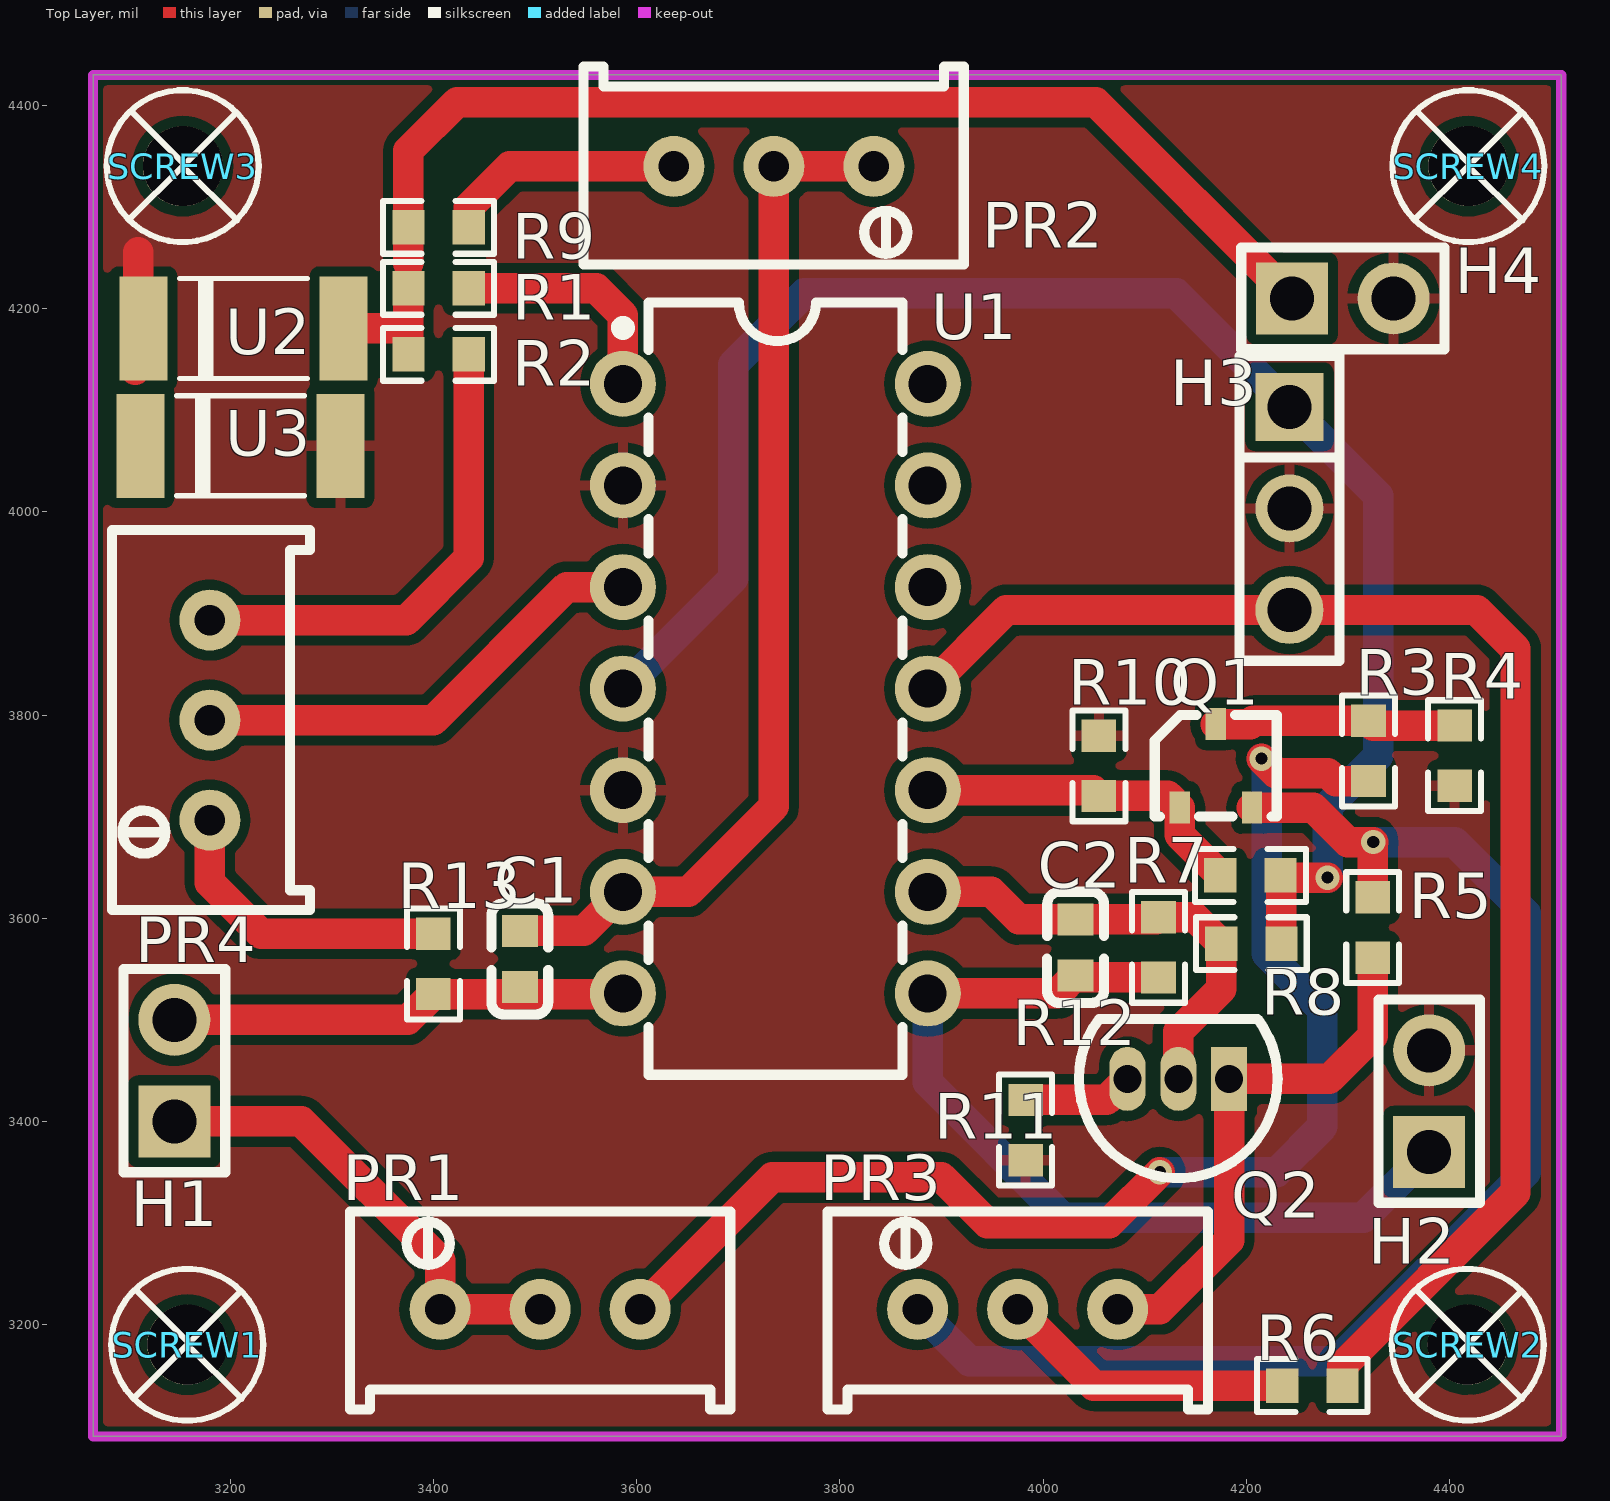
[diagram p0: Top Layer view]
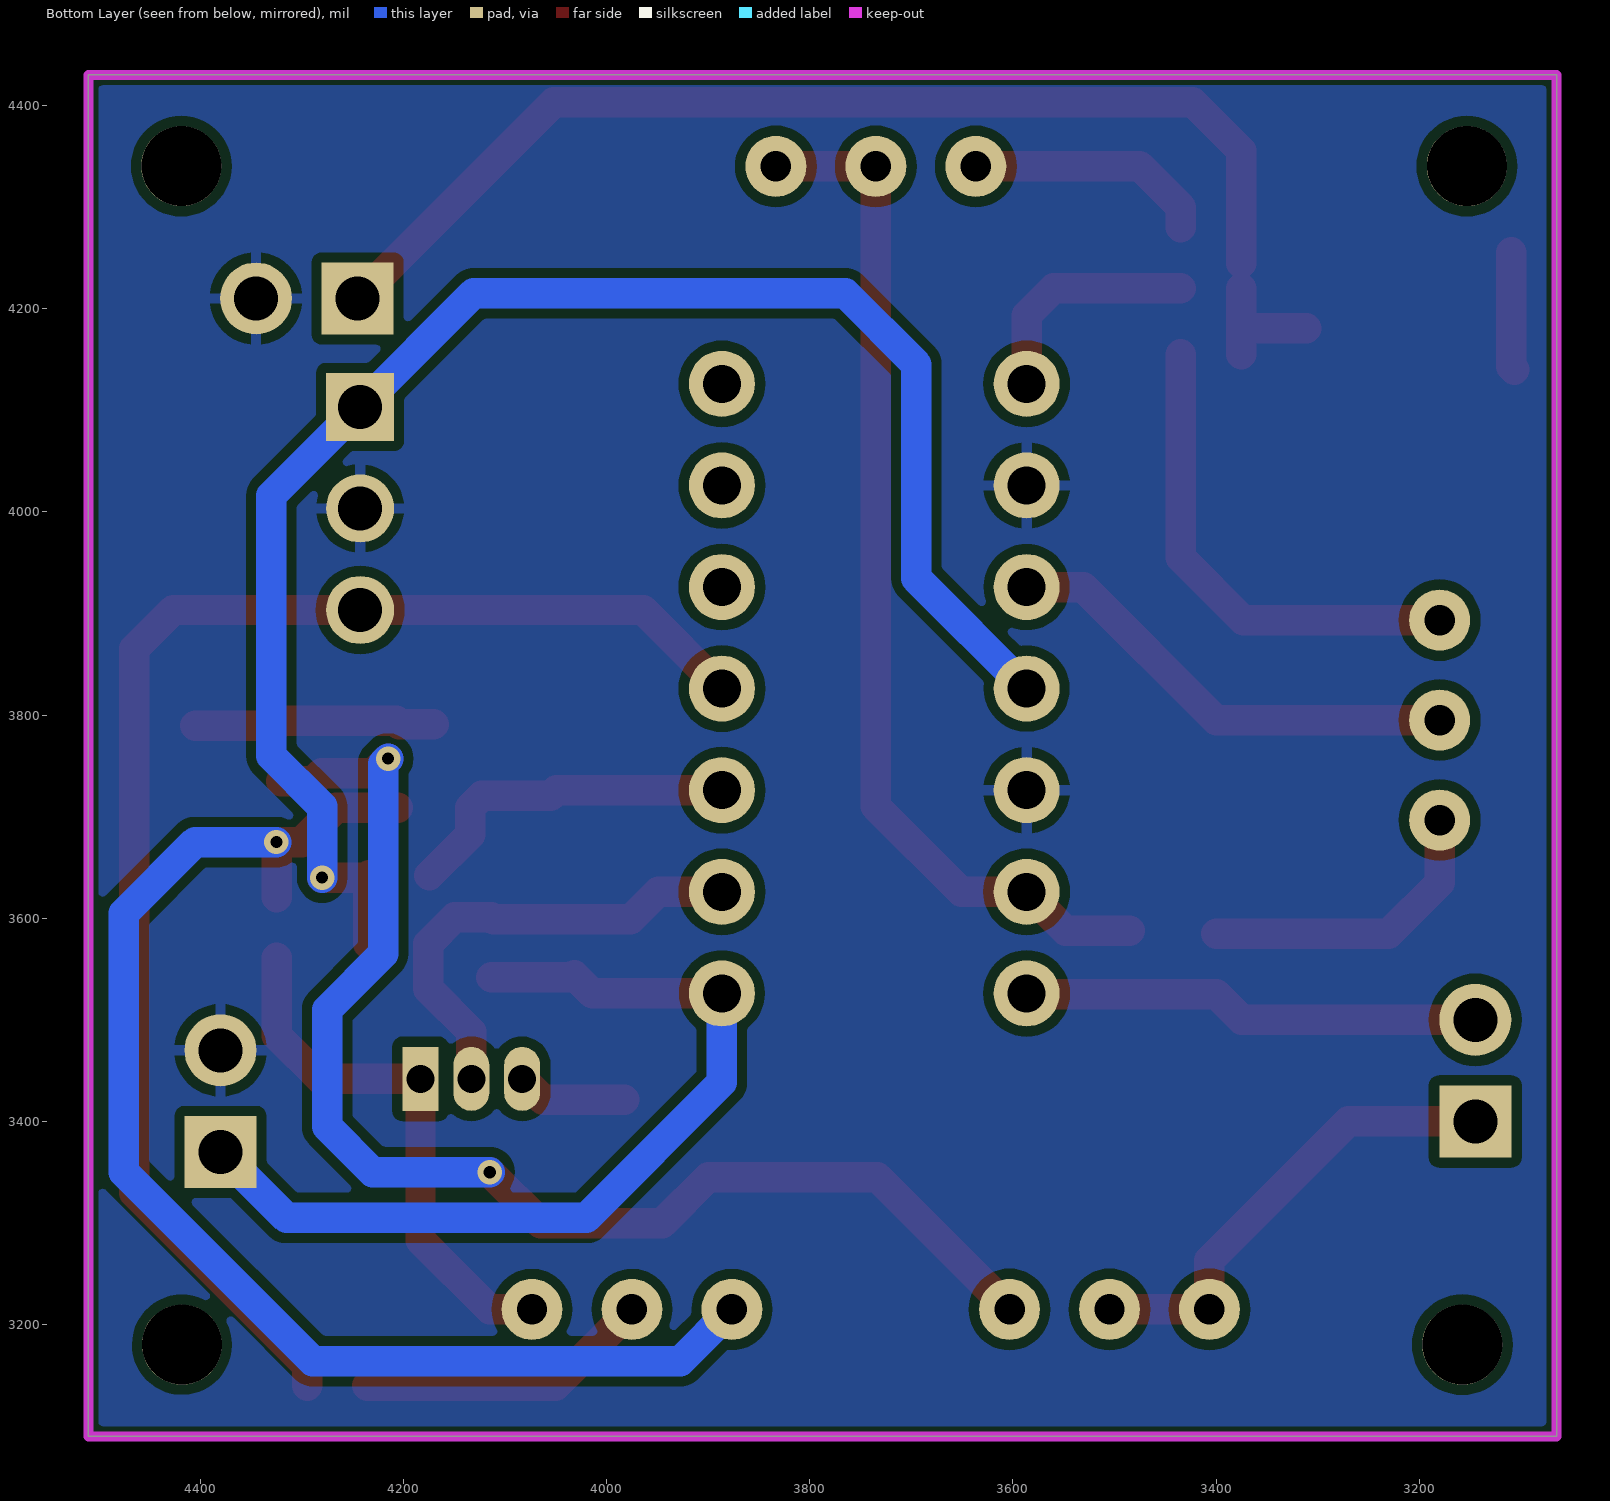
[diagram p1: Bottom Layer view, seen from below]
# Altium PCB MISC52119.pcbdoc
Units mil, origin at the board's own origin, x right, y up, seen from the top; angles counter-clockwise.
Board outline 1445 x 1340 mil, 2 copper layers (Top Layer, Bottom Layer), stack 62.206 mil thick; 32 components, 22 nets, 79 pads, 4 vias.

## Layer stack, top to bottom
Top Solder Mask Layer: solder mask 0.394, Dk 3.3
Top Layer: signal copper 1.379
Dielectric1: surface 59.449, FR4, Dk 4.5
Bottom Layer: signal copper 1.378
Bottom Solder Mask Layer: solder mask 0.394, Dk 3.3

## Board outline
3065,4430 3065,3090 4510,3090 4510,4430

## Design rules (kind name [scope] priority, off if disabled: settings)
BoardOutlineClearance copperThickness2oz_1 [All] p2 off: genericclearance=7.99 ignorepadtopadclearanceinfootprint=FALSE except(0: Arc-SplitContinuation Track-SplitContinuation SMDPad-SplitContinuation THPad-SplitContinuation Via-SplitContinuation Fill-SplitContinuation Region-SplitContinuation Poly-SplitContinuation Text-SplitContinuation Hole-SplitContinuation; 5.98: Arc-CutoutEdge SMDPad-CutoutEdge THPad-CutoutEdge Via-CutoutEdge Fill-CutoutEdge Region-CutoutEdge Text-CutoutEdge; 6.93: Hole-OutlineEdge Hole-CutoutEdge; 10: Poly-OutlineEdge Poly-CutoutEdge; 11.81: Arc-OutlineEdge Track-OutlineEdge SMDPad-OutlineEdge THPad-OutlineEdge Via-OutlineEdge Fill-OutlineEdge Region-OutlineEdge Text-OutlineEdge Track-CutoutEdge)
BoardOutlineClearance copperThickness1oz_1 [All] p4: genericclearance=4.02 ignorepadtopadclearanceinfootprint=FALSE except(0: Arc-SplitContinuation Track-SplitContinuation SMDPad-SplitContinuation THPad-SplitContinuation Via-SplitContinuation Fill-SplitContinuation Region-SplitContinuation Poly-SplitContinuation Text-SplitContinuation Hole-SplitContinuation; 6: SMDPad-CutoutEdge THPad-CutoutEdge Via-CutoutEdge Fill-CutoutEdge Region-CutoutEdge Text-CutoutEdge; 6.93: Hole-OutlineEdge Hole-CutoutEdge; 10: Poly-OutlineEdge Poly-CutoutEdge; 11.8: Arc-OutlineEdge Track-OutlineEdge SMDPad-OutlineEdge THPad-OutlineEdge Via-OutlineEdge Fill-OutlineEdge Region-OutlineEdge Text-OutlineEdge; 11.81: Arc-CutoutEdge Track-CutoutEdge)
Clearance copperThickness2oz [All] p1 off: gap=7.99 ignorepadtopadclearanceinfootprint=FALSE except(5.98: SMDPad-Track SMDPad-SMDPad THPad-Track SMDPad-THPad THPad-THPad Track-Via SMDPad-Via THPad-Via Via-Via Fill-Track Region-Track Fill-SMDPad Region-SMDPad Fill-THPad Region-THPad Fill-Via Region-Via Fill-Fill Fill-Region Region-Region Arc-Track Arc-SMDPad Arc-THPad Arc-Via Fill-Arc Region-Arc Arc-Arc Text-Track SMDPad-Text Text-THPad Text-Via Fill-Text Region-Text Arc-Text Text-Text; 6.93: Hole-Track Hole-SMDPad Hole-THPad Hole-Via Fill-Hole Region-Hole Hole-Arc Hole-Text; 10: Poly-Track Poly-SMDPad Poly-THPad Poly-Via Poly-Fill Poly-Region Poly-Poly Poly-Arc Poly-Text Poly-Hole)
Clearance copperThickness1oz [All] p3: gap=4.02 ignorepadtopadclearanceinfootprint=FALSE except(5.98: SMDPad-Track SMDPad-SMDPad THPad-Track SMDPad-THPad THPad-THPad Track-Via SMDPad-Via THPad-Via Via-Via Fill-Track Region-Track Fill-SMDPad Region-SMDPad Fill-THPad Region-THPad Fill-Via Region-Via Fill-Fill Fill-Region Region-Region; 6: Arc-Track Arc-SMDPad Arc-THPad Arc-Via Fill-Arc Region-Arc Arc-Arc Text-Track SMDPad-Text Text-THPad Text-Via Fill-Text Region-Text Arc-Text Text-Text; 6.93: Hole-Track Hole-SMDPad Hole-THPad Hole-Via Fill-Hole Region-Hole Hole-Arc Hole-Text; 10: Poly-Track Poly-SMDPad Poly-THPad Poly-Via Poly-Fill Poly-Region Poly-Poly Poly-Arc Poly-Text Poly-Hole)
DiffPairsRouting differentialPair [All] p1: maxlimit=6 minlimit=6 mostfreqgap=6 toplayer_minwidth=5 toplayer_prefwidth=10 toplayer_maxwidth=100 toplayer_mingap=6 toplayer_prefgap=6 toplayer_maxgap=6 bottomlayer_minwidth=5 bottomlayer_prefwidth=10 bottomlayer_maxwidth=100 bottomlayer_mingap=6 bottomlayer_prefgap=6 bottomlayer_maxgap=6 maxuncoupledlength=10
HoleToHoleClearance otherClearance [All] p1: gap=11.81 allowstackedmicrovias=TRUE
Length netLength [All] p1: minlimit=0 maxlimit=0
MatchedLengths netLengthTolerance [All] p1: tolerance=1000
PasteMaskExpansion pasteMaskExpansion [All] p1: expansion=0
PlaneConnect innerPlane [All] p1: planeconnectstyle=Relief reliefexpansion=20 reliefentries=4 reliefconductorwidth=10 reliefairgap=10
PolygonConnect copperRegion [(InNet('GND'))] p1: connectstyle=Relief reliefconductorwidth=10 reliefentries=4 polygonreliefangle="90 Angle" airgapwidth=10 via.connectstyle=Relief via.reliefconductorwidth=10 via.reliefentries=4 via.polygonreliefangle="90 Angle" via.airgapwidth=10
RoutingVias viaSize [All] p1: holewidth=12.01 width=24.02 viastyle="Through Hole" minholewidth=11.81 minwidth=19.68 maxholewidth=248.03 maxwidth=393.7
SolderMaskExpansion solderMaskExpansion [IsVia] p1: expansion=-1000 istentingtop=TRUE
SolderMaskExpansion solderMaskExpansion [All] p2: expansion=2 istentingtop=FALSE
Width copperThickness2oz_2 [All] p1 off: maxlimit=100 minlimit=8 preferedwidth=10
Width copperThickness1oz_2 [All] p2: maxlimit=100 minlimit=5 preferedwidth=10

## Components (designator, comment, footprint, x,y, rotation, side; value= is the part's Value field where it differs from the comment)
C1 "100nF" C0603 3485,3560 r90 top
C2 "100pF" C0603 4032,3571.34 r270 top
H1 "" HDR-TH_2P-P2.54-V-M-1 3145,3450 r90 top
H2 "" HDR-TH_2P-P2.54-V-M-1 4380,3420 r90 top
H3 "" HDR-TH_3P-P2.54-V-M 4242.52,4003.37 r270 top
H4 "" HDR-TH_2P-P2.54-V-M-1 4295,4210 r0 top
PR1 "10kΩ" R_3296 3505,3220 r0 top
PR2 "100kΩ" R_3296 3735,4335 r180 top
PR3 "500" R_3296 3975,3220 r0 top
PR4 "5kΩ" R_3296 3175,3795 r90 top
Q1 "2N222" SMD_3-L3.0-W2.5_JANTXV2N2222AUB 4170,3750 r0 top
Q2 "2N3391A" TO-92-3_L4.9-W3.7-P1.27-L 4133.13,3441.87 r180 top
R1 "1kΩ" R0603 3405,4220 r0 top
R2 "20kΩ" R0603 3405,4155 r0 top
R3 "2.2K" R0603 4320.34,3764.66 r90 top
R4 "220" R0603 4405,3760 r90 top
R5 "390" R0603 4324.42,3590.87 r270 top
R6 "20K" R0603 4265,3140 r180 top
R7 "4.7K" R0603 4204.08,3642.15 r0 top
R8 "4.7K" R0603 4205,3575 r0 top
R9 "4.7K" R0603 3405,4280 r0 top
R10 "4.7K" R0603 4055,3750 r270 top
R11 "220" R0603 3982.79,3391.53 r90 top
R12 "4.7K" R0603 4113.65,3571.34 r90 top
R13 "20kΩ" R0603 3400,3555 r270 top
SCREW1 "" M2螺丝 3157.7,3180.25 r0 top
SCREW2 "" M2螺丝 4417.98,3180.25 r0 top
SCREW3 "" M2螺丝 3153.27,4340.25 r0 top
SCREW4 "" M2螺丝 4418.56,4340.25 r0 top
U1 "LM324N/PB" PDIP-14_L19.2-W6.6-P2.54-LS7.6-BL 3736.51,3825.98 r270 top
U2 "稳压管474536VSMA" LL-41_L5.0-W2.5-RD 3212.99,4180.53 r0 top
U3 "稳压管474536VSMA" LL-41_L5.0-W2.5-RD 3210,4065 r0 top

## Footprints (in the part's own frame and the unit in brackets; to place one, negate y for a bottom-side part, rotate by r counter-clockwise, add the part's x,y. Pads: shape width x height; smd on the part's side, far side on the other; paste and mask are expansions set on the pad)
C0603 [mm]
  rect 0.8x0.9 smd: 1(-0.7,0) 2(0.7,0)
  silkscreen extent -1.39,-0.71 1.39,0.71
HDR-TH_2P-P2.54-V-M-1 [mm]
  rect 1.8x1.8 hole 1.1: 1(-1.27,0)
  round 1.8 hole 1.1: 2(1.27,0)
  silkscreen extent -2.54,-1.27 2.54,1.27
HDR-TH_3P-P2.54-V-M [mm]
  rect 1.7x1.7 hole 1.1: 1(-2.54,0)
  round 1.7 hole 1.1: 2(0,0) 3(2.54,0)
  silkscreen extent -3.81,-1.25 3.81,1.25
LL-41_L5.0-W2.5-RD [mm]
  rect 1.2x2.6 smd: 1(-2.5,0) 2(2.5,0)
  silkscreen extent -1.6,-1.25 1.6,1.25
M2螺丝 [mm]
  round 2 hole 2: 1(0,0)
  silkscreen extent -1.9,-1.9 1.9,1.9
PDIP-14_L19.2-W6.6-P2.54-LS7.6-BL [mm]
  round 1.65 hole 0.95: 1(-7.62,-3.81) 2(-5.08,-3.81) 3(-2.54,-3.81) 4(0,-3.81) 5(2.54,-3.81) 6(5.08,-3.81) 7(7.62,-3.81) 8(7.62,3.81) 9(5.08,3.81) 10(2.54,3.81) 11(0,3.81) 12(-2.54,3.81) 13(-5.08,3.81) 14(-7.62,3.81)
  silkscreen extent -9.65,-3.96 9.65,3.17
R0603 [mil]
  rect 31.75x34.02 smd paste-3937.01 mask+2: 1(-29.66,0) 2(29.66,0)
  silkscreen extent -55,-26 55,26
R_3296 [mil]
  round 60 hole 30 paste+0 mask+2: 1(-98.4,-5) 2(0,-5) 3(98.4,-5)
  silkscreen extent -187,-103 187,92
SMD_3-L3.0-W2.5_JANTXV2N2222AUB [mm]
  rect 0.51x0.8 smd: 1(-0.905,-1.045) 2(0.905,-1.045) 3(0,1.045)
  silkscreen extent -1.52,-1.27 1.52,1.27
TO-92-3_L4.9-W3.7-P1.27-L [mm]
  rect 0.9x1.6 hole 0.7: 1(-1.27,0)
  oval 0.9x1.6 hole 0.7: 2(0,0) 3(1.27,0)
  silkscreen extent -2.48,-1.5 2.48,2.48

## Via types
v1: diameter 24.02, hole 12, Top Layer to Bottom Layer, 4 vias

## Nets (pads, with @x,y where several pads share a name; then routed paths per layer and width w, separated by ;. In a path a pad name is that pad's centre, name@x,y a point inside that pad or via, vN(x,y) a via of type N, cw(c..) or ccw(c..) an arc to the next point about the centre after c; other vN are vias at no path point)
10V: H3.1 R7.2 R8.2 U1.4 | length 1620.4
  Top Layer w30: R7.2 R7.2@4234.66,3641.23 ; R8.2 R7.2@4234.66,3641.23 ; v1(4280,3640) 4235.89,3640 R7.2@4234.66,3641.23
  Bottom Layer w30: U1.4 3695,3934.46 3695,4145 3765,4215 4130.88,4215 H3.1 4330,4015.88 4330,3760 4280,3710 v1(4280,3640)
$1N1: PR4.3 R2.2 | length 480.4
  Top Layer w30: PR4.3 3373.4,3893.4 3434.66,3954.66 R2.2
$1N12: C1.2 PR2.1 PR2.2 U1.6 | length 1029.1
  Top Layer w30: C1.2 3548.1,3587.56 U1.6 3650.98,3625.98 3735,3710 PR2.2 PR2.1
$1N30: PR4.2 U1.3 | length 460.8
  Top Layer w30: PR4.2 3400,3795 3530.98,3925.98 U1.3
$1N31: R1.2 U1.1 | length 230.3
  Top Layer w30: R1.2 3560,4220 3586.52,4193.48 U1.1
$1N35: U2.1 U3.1 | length 116.8
  Top Layer w30: U2.1@3106.57,4140 3109.57,4142.99 3109.57,4255.53
$1N39: H1.1 PR1.1 PR1.2 | length 463.4
  Top Layer w30: H1.1 3270,3400 3406.6,3263.4 PR1.1@3406.6,3216.6 ; PR1.1 PR1.2
$1N40: PR1.3 R3.1 | length 1284.9
  Top Layer w30: PR1.3 3733.4,3345 3900,3345 3945,3300 4065,3300 v1(4115,3350) ; v1(4215,3757.13) 4229.25,3742.88 4280.23,3742.88 4288.11,3735 R3.1
  Bottom Layer w30: v1(4115,3350) 4230,3350 4275,3395 4275,3510 4220,3565 4220,3752.13 v1(4215,3757.13)
$1N41: Q1.3 R3.2 R4.2 | length 238.2
  Top Layer w30: Q1.3 4203.86,3791.14 4207.04,3794.32 R3.2 4325,3789.66 R4.2
$1N43: PR3.3 Q2.1 R5.2 | length 532.4
  Top Layer w30: PR3.3 4115,3215 4183.13,3283.13 Q2.1 4281.87,3441.87 4324.42,3484.42 R5.2
$1N44: PR3.1 Q1.2 R5.1 | length 1318.7
  Top Layer w30: Q1.2 4266.14,3708.86 4300,3675 v1(4325,3675) 4324.42,3674.42 R5.1
  Bottom Layer w30: PR3.1 3927.58,3164.02 4289.02,3164.02 4475,3350 4475,3605 4405,3675 v1(4325,3675)
$1N45: PR3.2 R6.2 | length 291.4
  Top Layer w30: PR3.2 4050,3140 R6.2
$1N47: Q1.1 R7.1 R10.2 U1.10 | length 338.2
  Top Layer w30: U1.10 4049.36,3725.98 R10.2 4122.89,3720.34 Q1.1 4134.37,3682.2 R7.1
$1N48: C2.1 Q2.2 R8.1 R12.2 U1.9 | length 462.3
  Top Layer w30: U1.9 3949.02,3625.98 3976.1,3598.9 C2.1 4111.55,3598.9 R12.2 4149.34,3601 R8.1 4175.34,3530.34 4133.13,3488.13 Q2.2
$1N51: Q2.3 R11.2 | length 108.9
  Top Layer w30: R11.2 4062.45,3421.19 Q2.3
$1N53: C2.2 H2.1 R12.1 U1.8 | length 898.6
  Top Layer w30: U1.8 4014.2,3525.98 C2.2 4034.1,3541.68 R12.1
  Bottom Layer w30: U1.8 3886.52,3438.48 4020,3305 4315,3305 H2.1
$1N55: C1.1 H1.2 R13.2 U1.7 | length 452.3
  Top Layer w30: H1.2 3374.66,3500 R13.2 3585.88,3525.34 U1.7
$1N56: PR4.1 R13.1 | length 302.5
  Top Layer w30: PR4.1 3180,3635 3230.34,3584.66 R13.1
$1N57: PR2.3 R9.2 | length 238.3
  Top Layer w30: R9.2 3434.66,4299.66 3475,4340 PR2.3
$1N58: H4.1 R1.1 R2.1 R9.1 U2.2 | length 1210.2
  Top Layer w30: U2.2 3373.19,4180.53 3375.34,4178.38 ; R2.1 3375.34,4178.38 ; R1.1 3375.34,4178.38 ; 3375.34,4244.45 R9.1 3375.34,4355.34 3423.2,4403.2 4051.8,4403.2 H4.1
-10V: H3.3 R6.1 U1.11 | length 1422
  Top Layer w30: U1.11 3963.9,3903.37 H3.3 4426.63,3903.37 4465,3865 4465,3330 4294.66,3159.66 R6.1
GND: H2.2 H3.2 H4.2 R4.1 R10.1 R11.1 U1.2 U1.5 U3.2
pads on no net: SCREW1.1 SCREW2.1 SCREW3.1 SCREW4.1 U1.12 U1.13 U1.14

## Polygon pours and split planes (outlines as drawn)
GND on Top Layer (solid, remove dead copper, pour order 0): 3000,4620 3000,3020 4560,3020 4560,4620
GND on Bottom Layer (solid, remove dead copper, pour order 2): 3020,4535 3020,3000 4570,3000 4570,4535

## Keep-outs
Board Outline Layer:
  the board outline again, w10